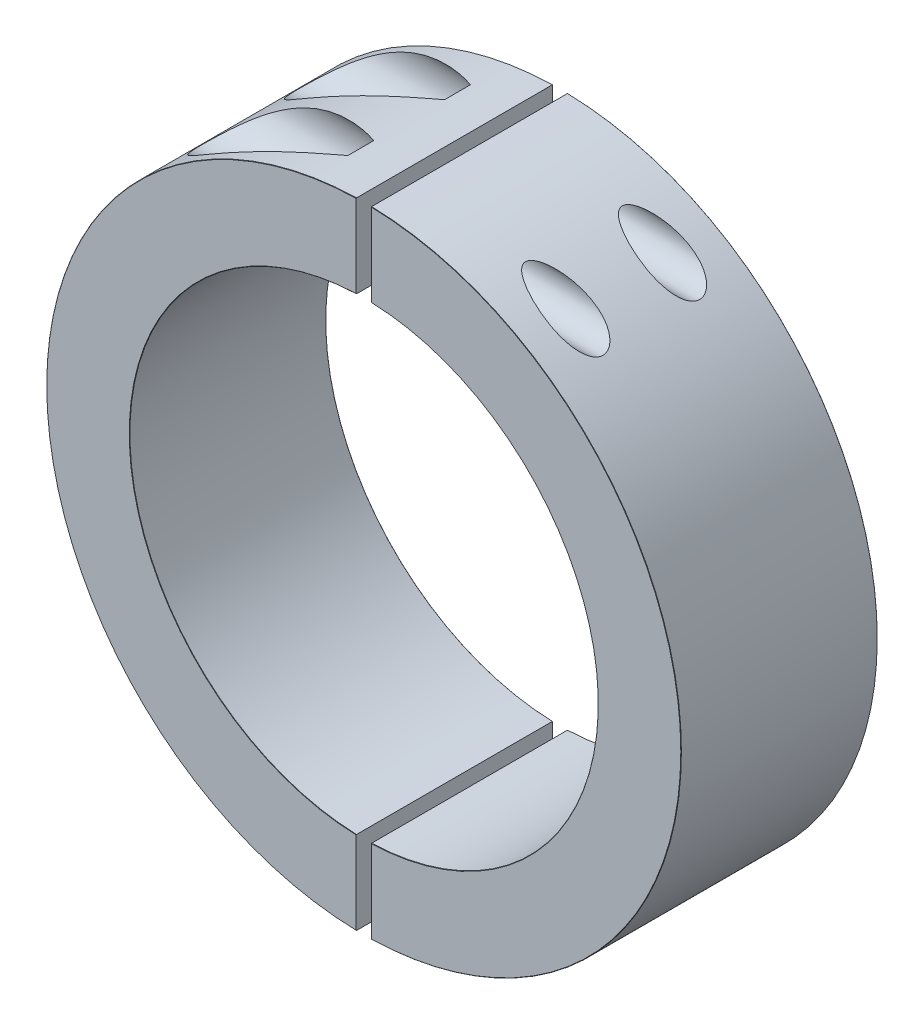
SolidWorks part; units mm, degrees
ref_plane "Front Plane" through (0, 0, 0) normal (0, 0, 1) x (1, 0, 0)
ref_plane "Top Plane" through (0, 0, 0) normal (0, 1, 0) x (1, 0, 0)
ref_plane "Right Plane" through (0, 0, 0) normal (1, 0, 0) x (0, 0, -1)
sketch "Sketch1" plane through (0, 0, 0) normal (0, 0, 1) x (1, 0, 0)
  circle A0 centre (0, 0) radius 105
  circle A1 centre (0, 0) radius 77.5
  dimension "D1" = 210
  dimension "D2" = 155
extrude "Boss-Extrude1" add sketch "Sketch1" along normal blind 65
cosmetic thread "Cosmetic Thread1" [suppressed] parameters "D2"=182
chamfer "Chamfer1" distance 0.1 angle 45 4 edges at (77.5, 0, 0) (77.5, 0, 65) (105, 0, 0) (105, 0, 65)
sketch "Sketch2" plane through (0, 0, 0) normal (0, 0, -1) x (-1, 0, 0)
  line L1 (-2.5, 145.451) -> (2.5, 145.451)
  line L2 (-2.5, 145.451) -> (-2.5, -145.451)
  line L3 (-2.5, -145.451) -> (2.5, -145.451)
  line L4 (2.5, 145.451) -> (2.5, -145.451)
  line L5 (-2.5, 145.451) -> (2.5, -145.451) construction
  line L6 (-2.5, -145.451) -> (2.5, 145.451) construction
  point P0 (0, 0)
  dimension "D1" = 5
extrude "Cut-Extrude1" cut sketch "Sketch2" against normal through all
sketch "Sketch3" plane through (-2.5, 0, 0) normal (1, 0, 0) x (0, 0, -1)
  line L0 (-82.2896, 91.25) -> (24.0887, 91.25) construction
  line L1 (-32.5, 104.9702) -> (-32.5, 26.6974) construction
  line L2 (-0.1, 104.9702) -> (-64.9, 104.9702) construction
  line L3 (-48.5, 104.9702) -> (-48.5, 26.6974) construction
  line L4 (-16.5, 104.9702) -> (-16.5, 26.6974) construction
  circle A0 centre (-48.5, 91.25) radius 13
  circle A1 centre (-16.5, 91.25) radius 13
  dimension "D3" = 26
  dimension "D4" = 26
  dimension "D5" = 91.25
  dimension "D1" = 16
  dimension "D2" = 16
extrude "Cut-Extrude2" cut sketch "Sketch3" against normal through all from offset 15 offset against normal yes
sketch "Sketch4" plane through (-17.5, 0, 0) normal (-1, 0, 0) x (0, 0, 1)
  circle A0 centre (48.5, 91.25) radius 8.5
  circle A1 centre (16.5, 91.25) radius 8.5
  dimension "D1" = 17
  dimension "D2" = 17
extrude "Cut-Extrude3" cut sketch "Sketch4" against normal blind 16
sketch "Sketch5" plane through (2.5, 0, 0) normal (-1, 0, 0) x (0, 0, 1)
  circle A0 centre (48.5, 91.25) radius 8
  circle A1 centre (16.5, 91.25) radius 8
hole_wizard "M16 Tapped Hole1" positions "Sketch6" profile "Sketch7" tap size "M16" standard "GB" end condition through all
sketch "Sketch6" plane through (2.5, 0, 0) normal (-1, 0, 0) x (0, 0, 1)
  point P0 (48.5, 91.25)
  point P3 (16.5, 91.25)
sketch "Sketch7" plane through (2.5, 91.25, 48.5) normal (0, 1, 0) x (0, 0, 1)
  line L0 (0, 0) -> (0, 102.5)
  line L1 (0, 102.5) -> (7, 102.5)
  line L2 (7, 102.5) -> (7, 0)
  line L5 (7, 0) -> (0, 0)
  line L11 (0, -6.35) -> (0, 107.95) construction
  dimension "通孔螺纹孔钻头直径" = 14
  dimension "通孔螺纹孔钻头深度" = 102.5
cosmetic thread "Cosmetic thread 1" parameters "D2"=16
cosmetic thread "Cosmetic thread 2" parameters "D2"=16
mirror "Mirror1" about plane through (0, 0, 0) normal (0, 1, 0) of "M16 Tapped Hole1"
mirror "Mirror2" about plane through (0, 0, 0) normal (0, 1, 0) of "Cut-Extrude2"
mirror "Mirror3" about plane through (0, 0, 0) normal (0, 1, 0) of "Cut-Extrude3"
sketch "Sketch9" plane through (0, 0, 0) normal (0, 0, -1) x (-1, 0, 0)
  circle A0 centre (0, 0) radius 85
  dimension "D1" = 170
extrude "Cut-Extrude4" [suppressed] cut sketch "Sketch9" against normal blind 5
